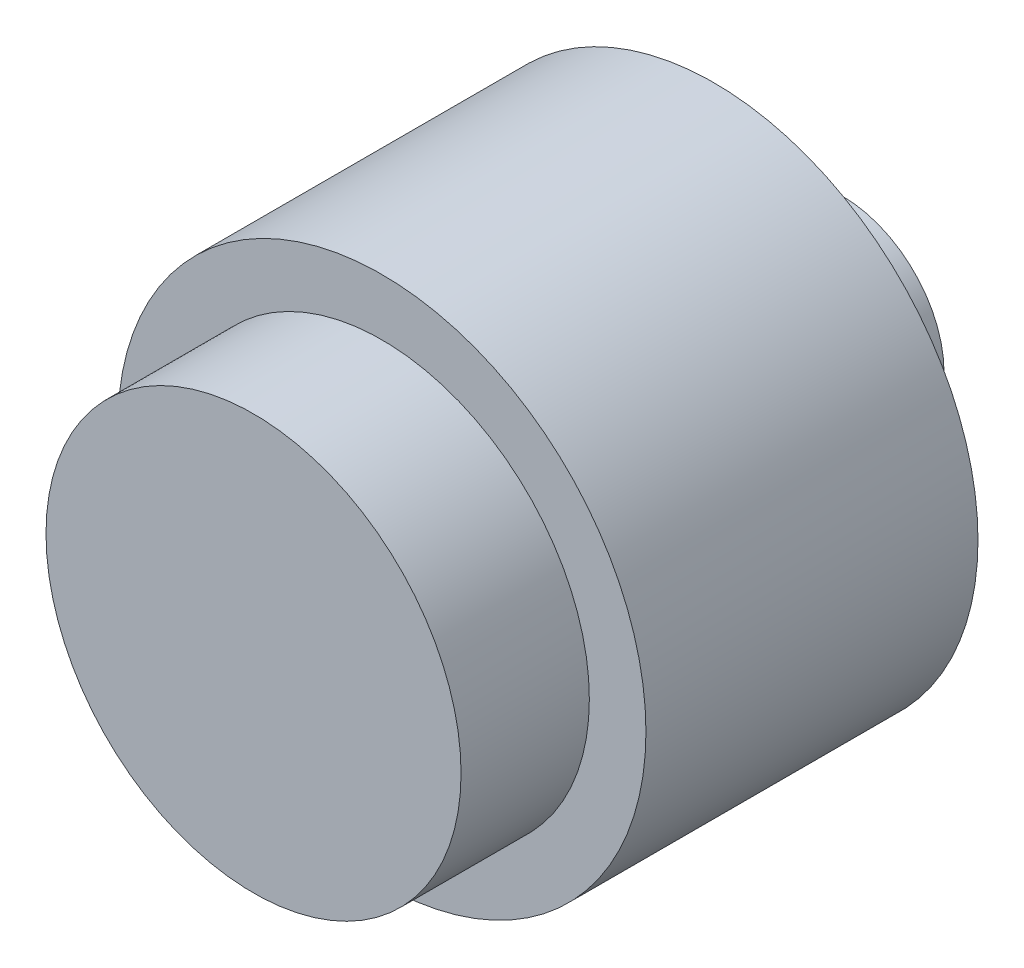
SolidWorks part; units mm, degrees
material "普通碳钢"
ref_plane "Front Plane" through (0, 0, 0) normal (0, 0, 1) x (1, 0, 0)
ref_plane "Top Plane" through (0, 0, 0) normal (0, 1, 0) x (1, 0, 0)
ref_plane "Right Plane" through (0, 0, 0) normal (1, 0, 0) x (0, 0, -1)
sketch "Sketch1" plane through (0, 0, 0) normal (0, 0, 1) x (1, 0, 0)
  circle A0 centre (0, 0) radius 27
  dimension "D1" = 54
extrude "Boss-Extrude1" add sketch "Sketch1" along normal blind 34
sketch "Sketch2" plane through (0, 0, 34) normal (0, 0, 1) x (1, 0, 0)
  circle A0 centre (0, 0) radius 70
  dimension "D1" = 140
extrude "Boss-Extrude2" add sketch "Sketch2" along normal blind 88
sketch "Sketch3" plane through (0, 0, 122) normal (0, 0, 1) x (1, 0, 0)
  circle A0 centre (0, 0) radius 55
  dimension "D1" = 110
extrude "Boss-Extrude3" add sketch "Sketch3" along normal blind 34
